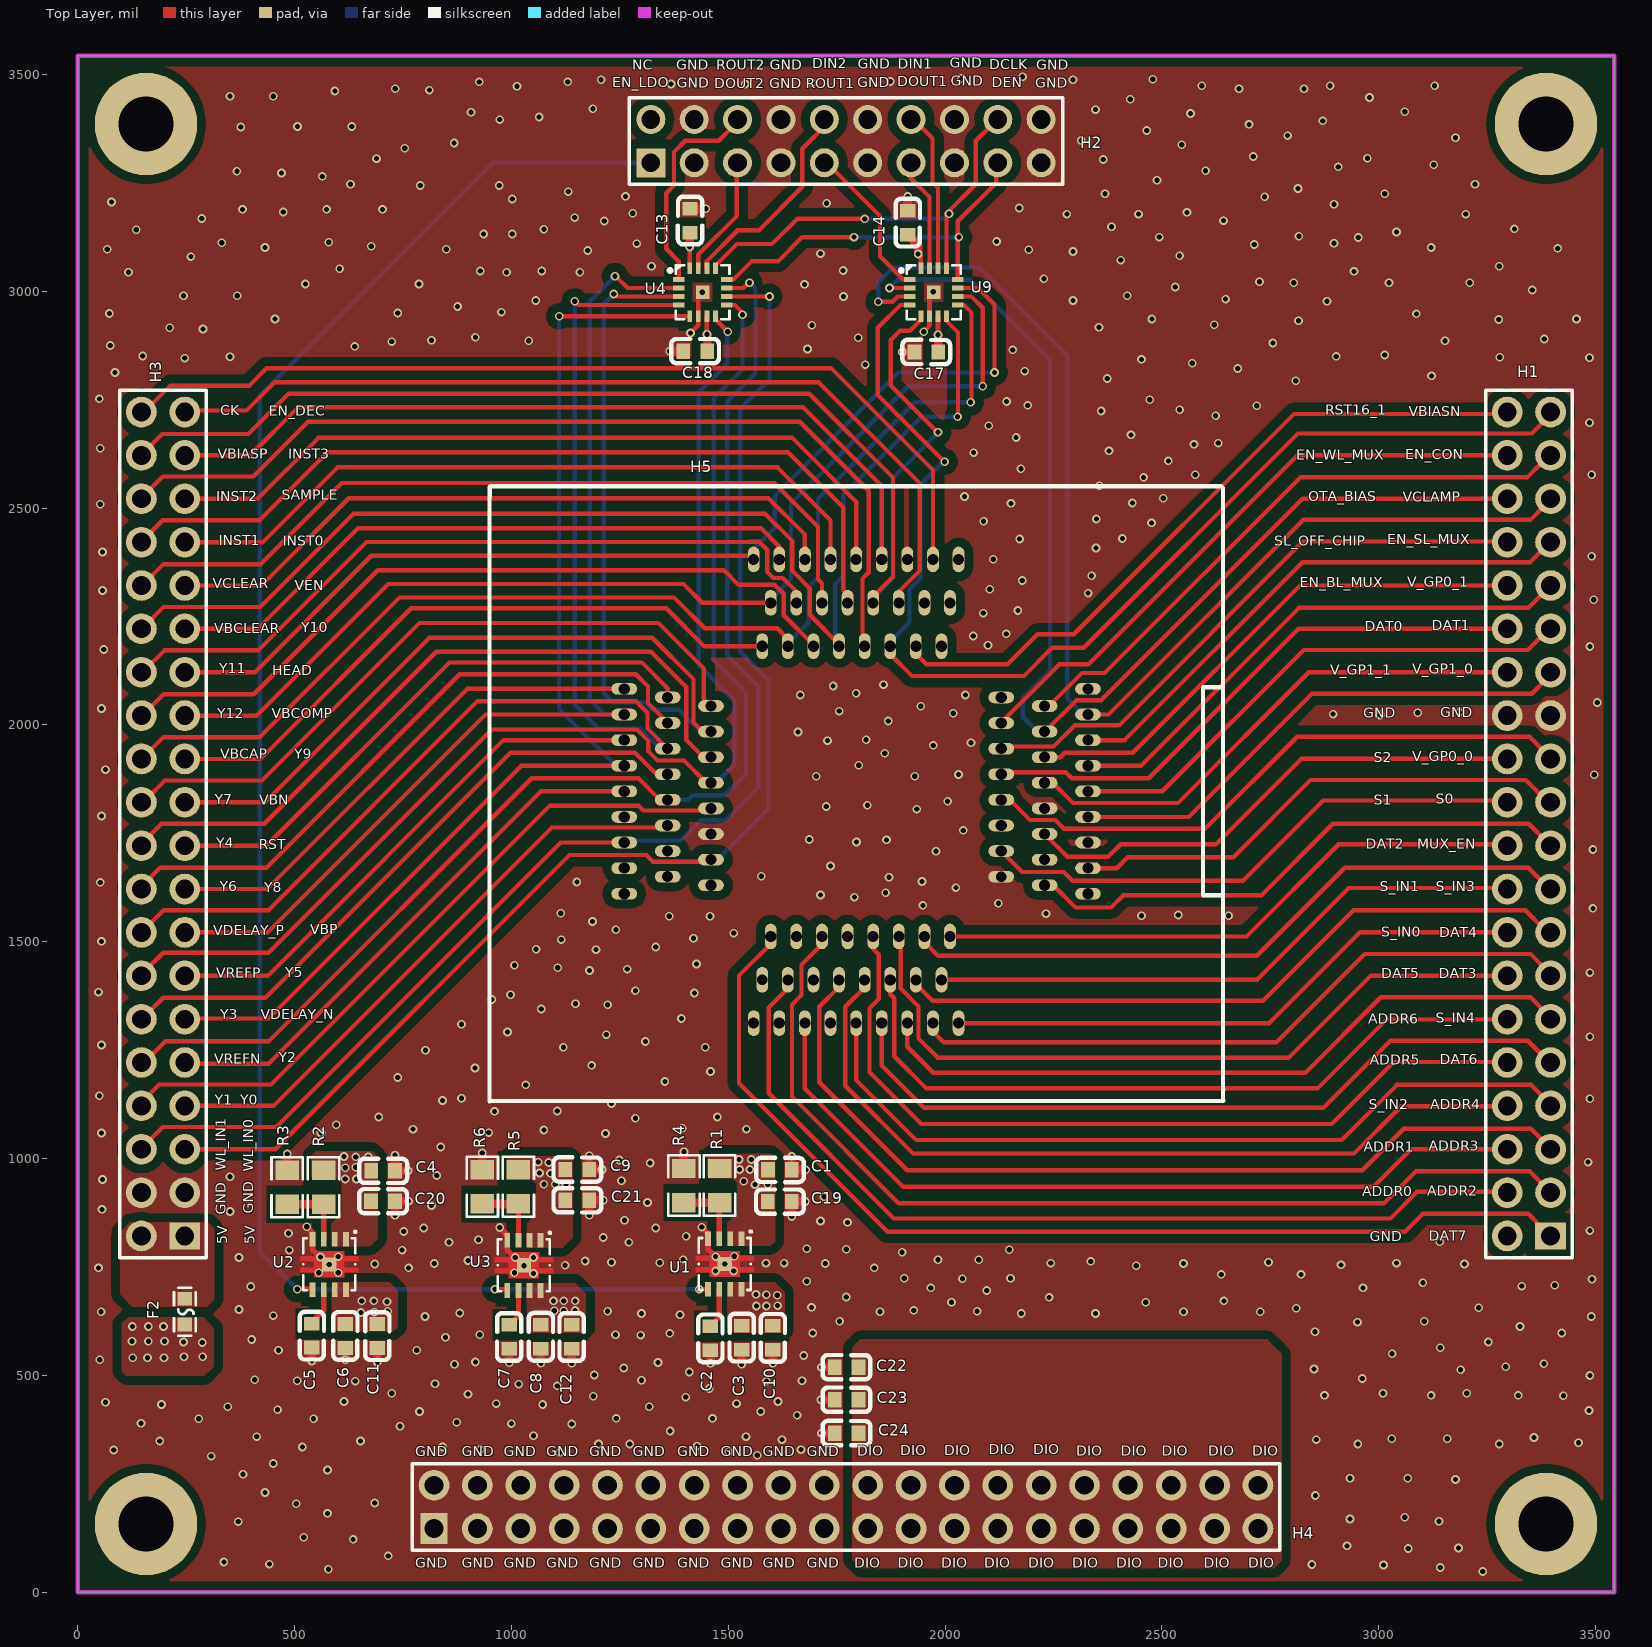
[diagram p0: Top Layer view]
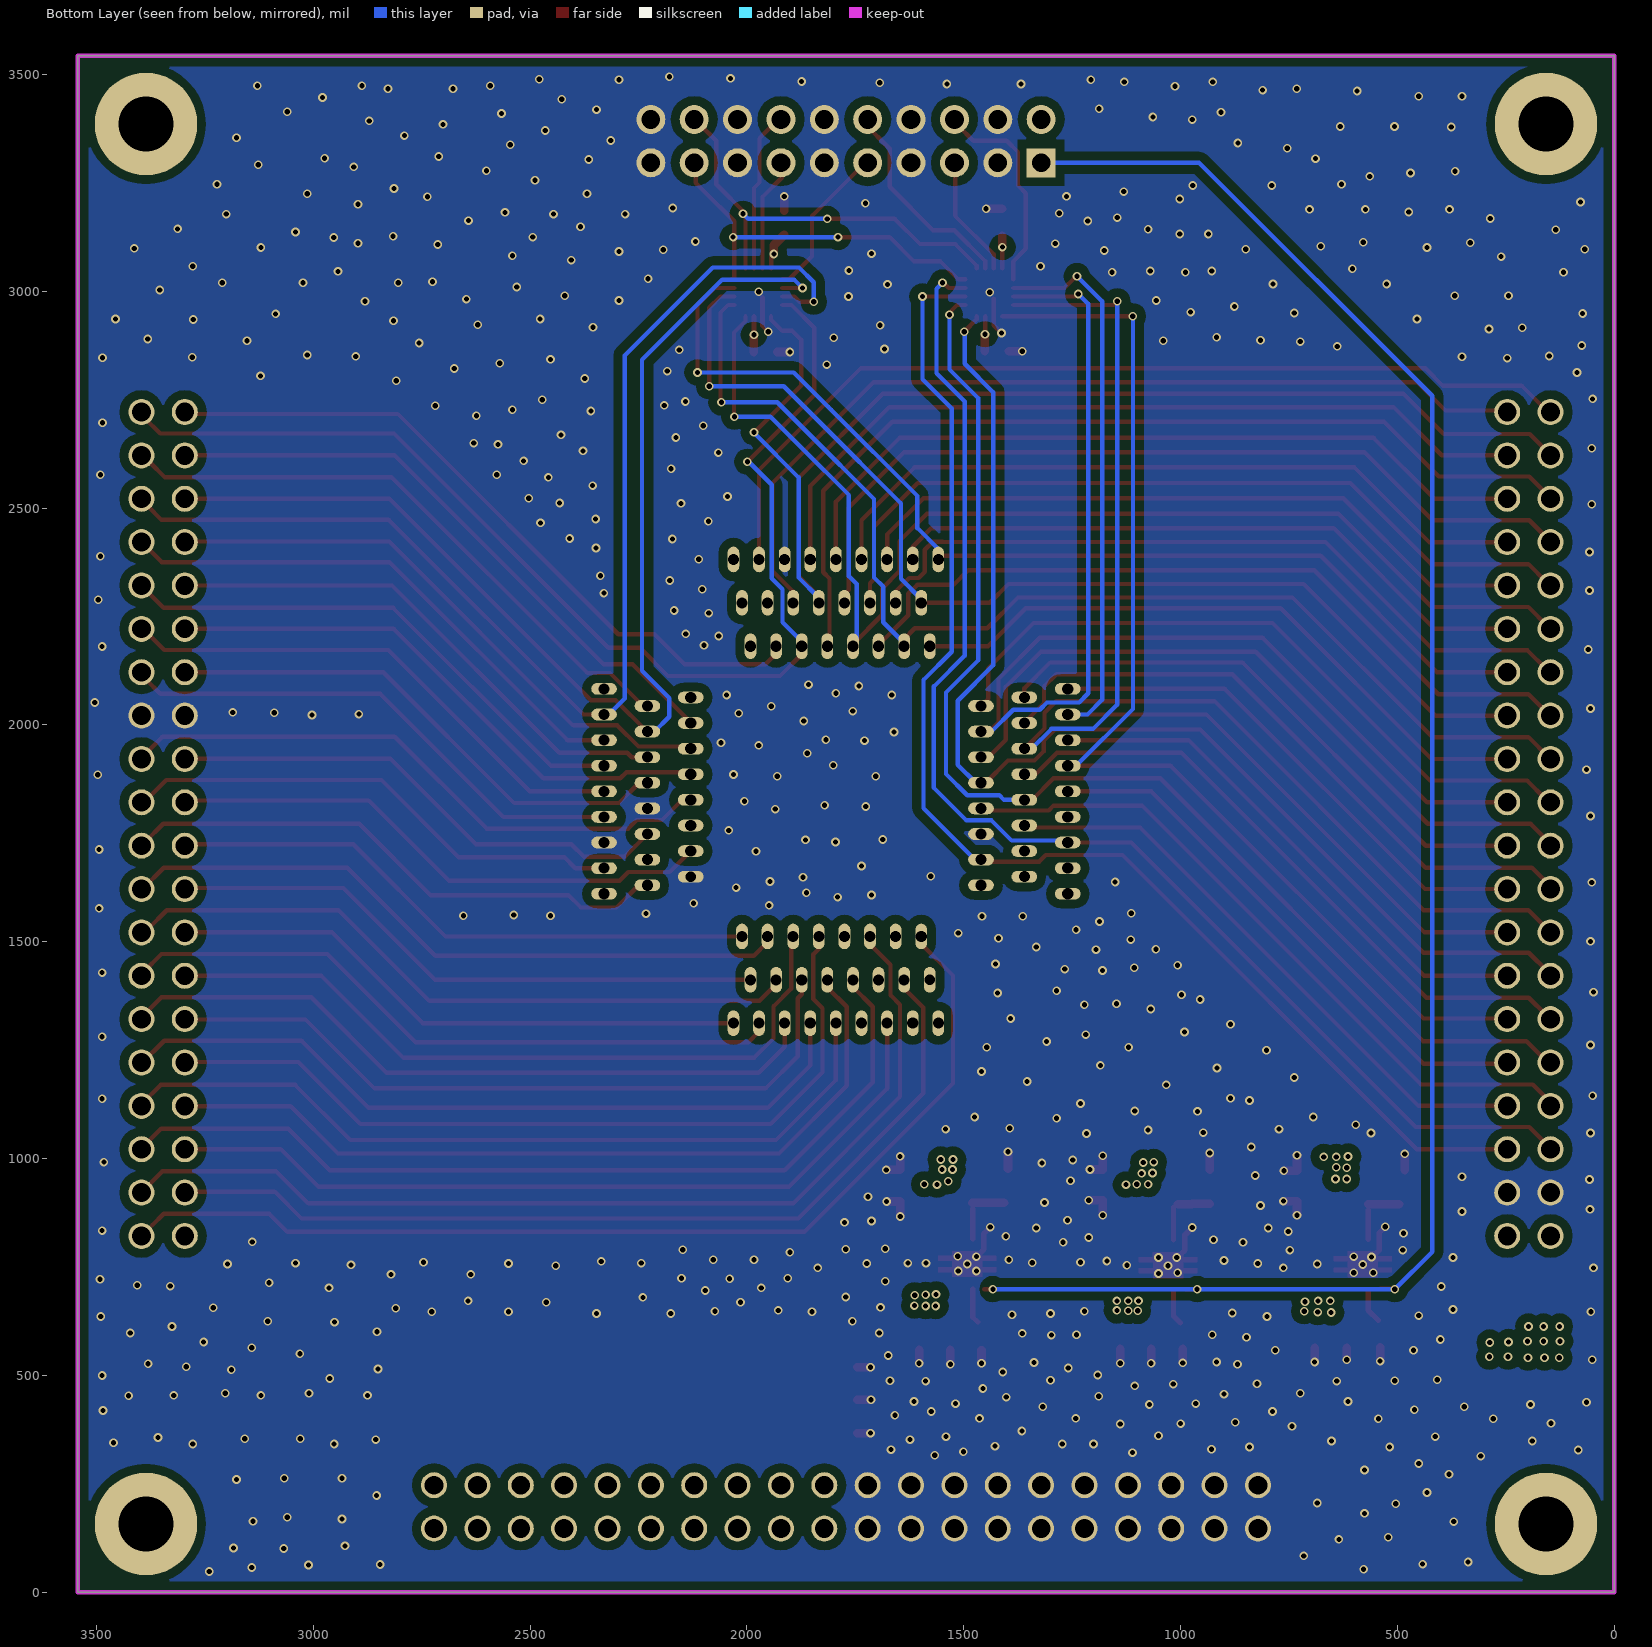
[diagram p1: Bottom Layer view, seen from below]
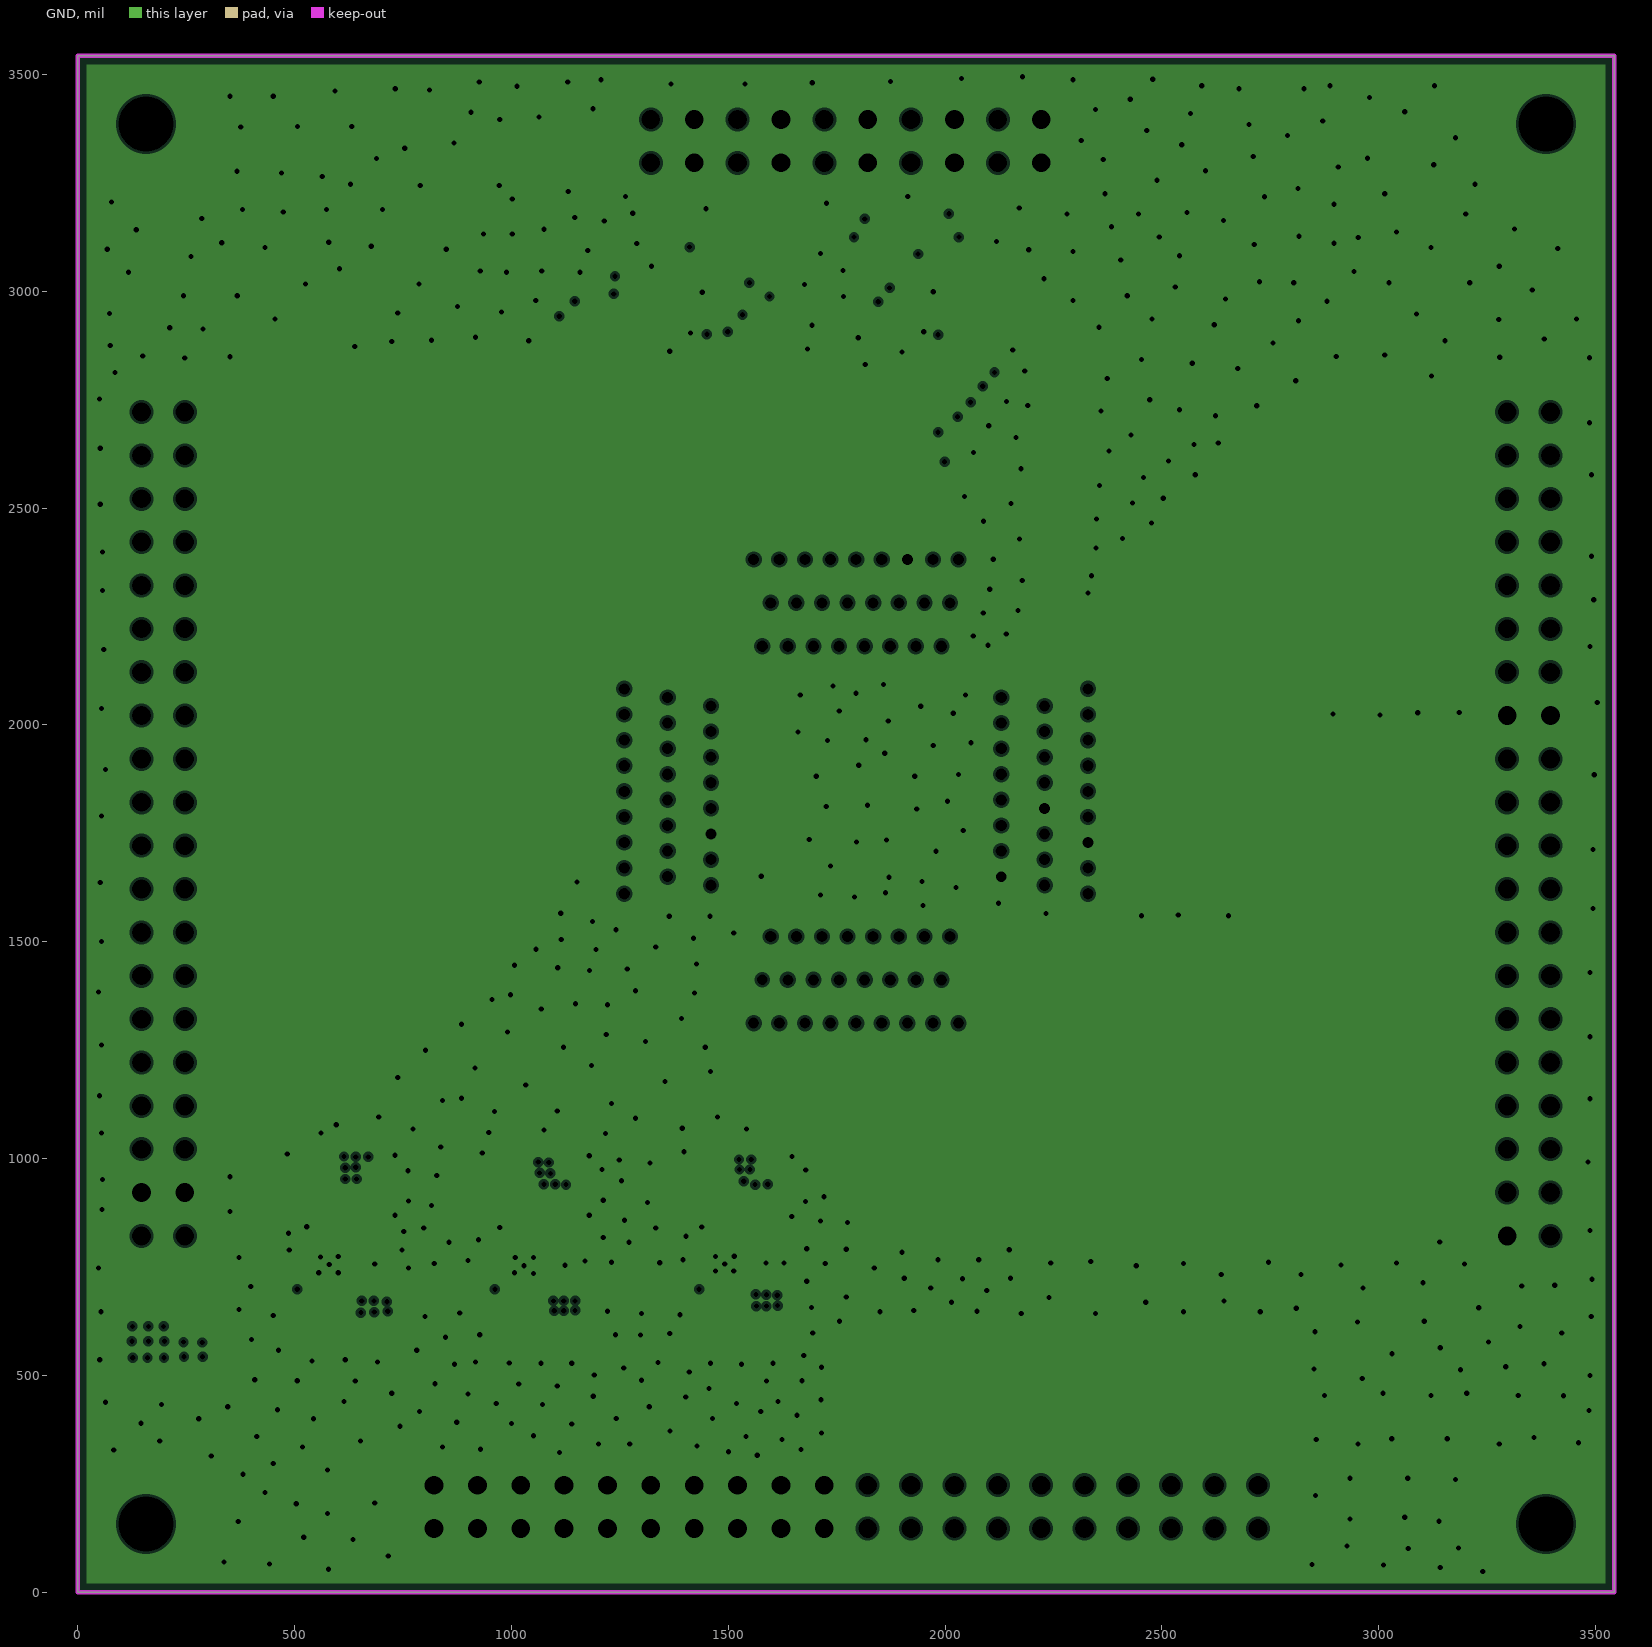
[diagram p2: GND, clearances drawn from the general rule]
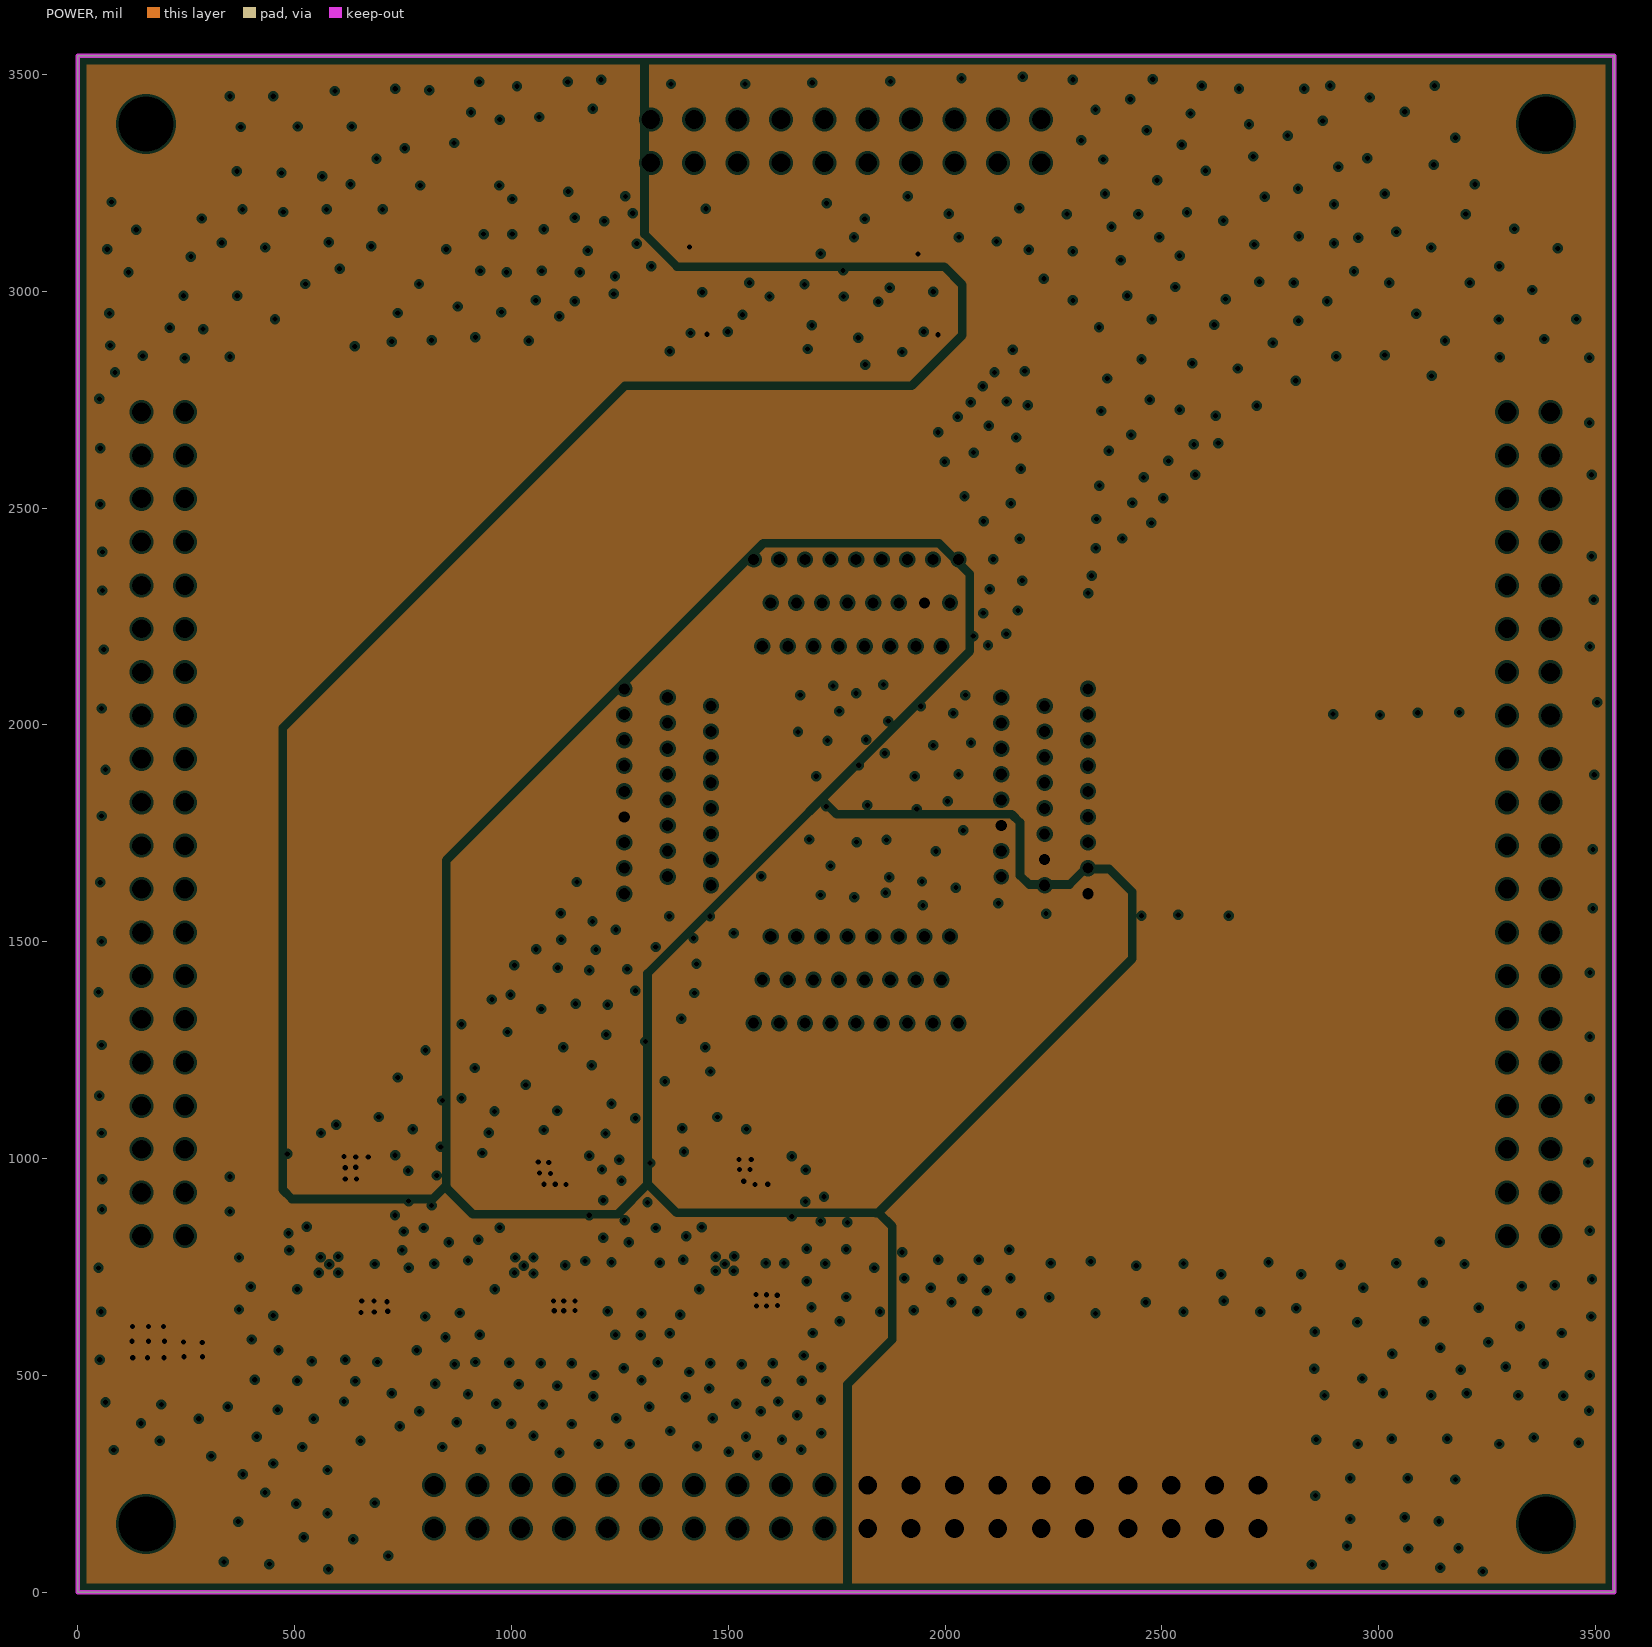
[diagram p3: POWER, clearances drawn from the general rule]
# Altium PCB MISC62795.pcbdoc (part 1 of 2)
Units mil, origin at the board's own origin, x right, y up, seen from the top; angles counter-clockwise.
Board outline 3543.31 x 3543.31 mil, 4 copper layers (Top Layer, GND, POWER, Bottom Layer); 39 components, 94 nets, 363 pads, 705 vias.

## Layer stack, top to bottom (the 12.6 mil dielectric is the usual default, probably not edited)
Top Layer: signal copper 1.4
Dielectric: core 12.6, FR-4, Dk 4.8
GND: plane copper 1.4, net GND
Dielectric: prepreg 12.6, FR-4, Dk 4.8
POWER: plane copper 1.4, net DVDDIO
Dielectric: core 12.6, FR-4, Dk 4.8
Bottom Layer: signal copper 1.4

## Board outline
0,0 3543.31,0 3543.31,3543.31 0,3543.31

## Design rules (kind name [scope] priority, off if disabled: settings)
Clearance Clearance_1 [INPOLYGON] p1: gap=6
Clearance [All] p2: gap=6
HoleSize [All] p1: absolutevalues=TRUE maxlimit=500 minlimit=1 maxpercent=80.000 minpercent=20.000
HoleToHoleClearance [All] p1: gap=0 allowstackedmicrovias=TRUE
MinimumSolderMaskSliver [All] p1: minsoldermaskwidth=0
PlaneClearance [All] p1: clearance=6
PlaneConnect [All] p1: planeconnectstyle=Direct reliefexpansion=20 reliefentries=4 reliefconductorwidth=10 reliefairgap=10
PolygonConnect [All] p1: connectstyle=Direct reliefconductorwidth=10 reliefentries=4 polygonreliefangle="90 Angle"
RoutingVias [All] p1: holewidth=12 width=20 viastyle="Through Hole" minholewidth=12 minwidth=20 maxholewidth=12 maxwidth=20
SilkToSilkClearance [All] p1: silktosilkclearance=0
SilkscreenOverComponentPads [All] p1: minsilkscreentomaskgap=0
SolderMaskExpansion [All] p1: expansion=4
Width [All] p1: maxlimit=40 minlimit=10 preferedwidth=10 minimp=50.000000 maximp=50.000000 favimp=50.000000
21 further rules are at their usual default settings.

## Components (designator, comment, footprint, x,y, rotation, side; value= is the part's Value field where it differs from the comment)
C1 "4.7uF/16V" C0603 1619.26,974.06 r180 top
C2 "10nF/16V" C0603 1459,586 r90 top
C3 "1uF/16V" C0603 1531,587 r270 top
C4 "4.7uF/16V" C0603 704.26,972.06 r180 top
C5 "10nF/16V" C0603 540,592 r90 top
C6 "1uF/16V" C0603 617,591 r270 top
C7 "10nF/16V" C0603 995,589 r90 top
C8 "1uF/16V" C0603 1068,589 r270 top
C9 "4.7uF/16V" C0603 1152,975 r180 top
C10 "4.7uF/16V" C0603 1603,587 r90 top
C11 "4.7uF/16V" C0603 691,591 r90 top
C12 "4.7uF/16V" C0603 1139,589 r90 top
C13 "0.1uF/16V" C0603 1412,3163 r270 top
C14 "0.1uF/16V" C0603 1914,3158 r270 top
C17 "0.1uF/16V" C0603 1957,2860 r0 top
C18 "0.1uF/16V" C0603 1424,2862 r0 top
C19 "4.7uF/16V" C0603 1619,901 r180 top
C20 "4.7uF/16V" C0603 704,902 r180 top
C21 "4.7uF/16V" C0603 1152,904 r180 top
C22 "4.7uF/16V" C0603 1773,519 r0 top
C23 "4.7uF/16V" C0603 1773,444 r0 top
C24 "4.7uF/16V" C0603 1773,367 r0 top
F2 "BSMD0603-050-6V" F0603 247,647 r90 top
H1 "12251220ANG0S115001" HDR-TH_40P-P2.54-V-M-R2-C20-S2.54 3346.46,1771.65 r90 top locked
H2 "PZ254V-12-20P" HDR-TH_20P-P2.54-V-M-R2-C10-S2.54 1771.65,3346.46 r0 top locked
H3 "12251220ANG0S115001" HDR-TH_40P-P2.54-V-M-R2-C20-S2.54 196.85,1771.65 r90 top locked
H4 "12251220ANG0S115001" HDR-TH_40P-P2.54-V-M-R2-C20-S2.54 1771.65,196.85 r0 top locked
H5 "220-1S-2*50PStraight row of mothersH=4.3 Gold-plated" IC51-1004-809-23 1795,1847 r90 top locked
R1 "1.25k" R0805 1480,938 r270 top
R2 "12.4k" R0805 567,934 r270 top
R3 "10k" R0805 483,934 r270 top
R4 "10k" R0805 1398,938 r270 top
R5 "12.4k" R0805 1016,935 r270 top
R6 "10k" R0805 933,935 r270 top
U1 "TPS7A8001DRBR" VSON-8_L3.0-W3.0-P0.65-TL-EP 1492,757 r270 top
U2 "TPS7A8001DRBR" VSON-8_L3.0-W3.0-P0.65-TL-EP 580,756 r270 top
U3 "TPS7A8001DRBR" VSON-8_L3.0-W3.0-P0.65-TL-EP 1029,754 r270 top
U4 "DAC60508ZRTER" WQFN-16_L3.0-W3.0-P0.50-BL-EP0.8 1441,2998 r270 top
U9 "DAC60508ZRTER" WQFN-16_L3.0-W3.0-P0.50-BL-EP0.8 1974,2998 r270 top

## Footprints (in the part's own frame and the unit in brackets; to place one, negate y for a bottom-side part, rotate by r counter-clockwise, add the part's x,y. Pads: shape width x height; smd on the part's side, far side on the other; paste and mask are expansions set on the pad)
C0603 [mm]
  rect 0.8x0.9 smd paste+0 mask+0.051: 1(-0.7,0) 2(0.7,0)
  silkscreen extent -1.41,-0.71 1.39,0.72
F0603 [mil]
  rect 31.75x34.02 smd paste-3937.01 mask+2: 1(-29.65,0) 2(29.66,0)
  silkscreen extent -55,-25 55,25
HDR-TH_20P-P2.54-V-M-R2-C10-S2.54 [mm]
  rect 1.7x1.7 hole 1.1 paste+0 mask+0.051: 1(-11.43,-1.27)
  round 1.7 hole 1.1 paste+0 mask+0.051: 2(-11.43,1.27) 3(-8.89,-1.27) 4(-8.89,1.27) 5(-6.35,-1.27) 6(-6.35,1.27) 7(-3.81,-1.27) 8(-3.81,1.27) 9(-1.27,-1.27) 10(-1.27,1.27) 11(1.27,-1.27) 12(1.27,1.27) 13(3.81,-1.27) 14(3.81,1.27) 15(6.35,-1.27) 16(6.35,1.27) 17(8.89,-1.27) 18(8.89,1.27) 19(11.43,-1.27) 20(11.43,1.27)
  silkscreen extent -12.7,-2.54 12.7,2.54
HDR-TH_40P-P2.54-V-M-R2-C20-S2.54 [mm]
  rect 1.575x1.8 / inner round 1.524 / far side round 1.524 hole 1.1: 1(-24.13,-1.27)
  round 1.8 / inner round 1.524 / far side round 1.524 hole 1.1: 2(-24.13,1.27) 3(-21.59,-1.27) 4(-21.59,1.27) 5(-19.05,-1.27) 6(-19.05,1.27) 7(-16.51,-1.27) 8(-16.51,1.27) 9(-13.97,-1.27) 10(-13.97,1.27) 11(-11.43,-1.27) 12(-11.43,1.27) 13(-8.89,-1.27) 14(-8.89,1.27) 15(-6.35,-1.27) 16(-6.35,1.27) 17(-3.81,-1.27) 18(-3.81,1.27) 19(-1.27,-1.27) 20(-1.27,1.27) 21(1.27,-1.27) 22(1.27,1.27) 23(3.81,-1.27) 24(3.81,1.27) 25(6.35,-1.27) 26(6.35,1.27) 27(8.89,-1.27) 28(8.89,1.27) 29(11.43,-1.27) 30(11.43,1.27) 31(13.97,-1.27) 32(13.97,1.27) 33(16.51,-1.27) 34(16.51,1.27) 35(19.05,-1.27) 36(19.05,1.27) 37(21.59,-1.27) 38(21.59,1.27) 39(24.13,-1.27) 40(24.13,1.27)
  silkscreen extent -25.4,-2.54 25.4,2.54
IC51-1004-809-23 [mm] "测试座"
  oval 1.5x0.686 hole 0.65: 1(-13.58,6) 3(-8.5,5) 4(-13.58,4.5) 5(-11.04,4) 6(-8.5,3.5) 7(-13.58,3) 8(-11.04,2.5) 9(-8.5,2) 10(-13.58,1.5) 11(-11.04,1) 12(-8.5,0.5) 13(-13.58,0) 14(-11.04,-0.5) 15(-8.5,-1) 16(-13.58,-1.5) 17(-11.04,-2) 18(-8.5,-2.5) 19(-13.58,-3) 20(-11.04,-3.5) 21(-8.5,-4) 22(-13.58,-4.5) 23(-11.04,-5) 24(-8.5,-5.5) 25(-13.58,-6) 51(13.58,-6) 52(11.04,-5.5) 53(8.5,-5) 54(13.58,-4.5) 55(11.04,-4) 56(8.5,-3.5) 57(13.58,-3) 58(11.04,-2.5) 59(8.5,-2) 60(13.58,-1.5) 61(11.04,-1) 62(8.5,-0.5) 63(13.58,0) 64(11.04,0.5) 65(8.5,1) 66(13.58,1.5) 67(11.04,2) 68(8.5,2.5) 69(13.58,3) 70(11.04,3.5) 71(8.5,4) 72(13.58,4.5) 73(11.04,5) 74(8.5,5.5) 75(13.58,6)
  oval 1.5x0.686 hole 0.61: 2(-11.04,5.5)
  oval 0.686x1.5 hole 0.65: 26(-6,-13.58) 27(-5.5,-11.04) 29(-4.5,-13.58) 30(-4,-11.04) 31(-3.5,-8.5) 32(-3,-13.58) 33(-2.5,-11.04) 34(-2,-8.5) 35(-1.5,-13.58) 36(-1,-11.04) 37(-0.5,-8.5) 38(0,-13.58) 39(0.5,-11.04) 40(1,-8.5) 41(1.5,-13.58) 42(2,-11.04) 43(2.5,-8.5) 44(3,-13.58) 45(3.5,-11.04) 46(4,-8.5) 47(4.5,-13.58) 48(5,-11.04) 49(5.5,-8.5) 50(6,-13.58) 76(6,13.58) 77(5.5,11.04) 78(5,8.5) 79(4.5,13.58) 80(4,11.04) 81(3.5,8.5) 82(3,13.58) 83(2.5,11.04) 84(2,8.5) 85(1.5,13.58) 86(1,11.04) 87(0.5,8.5) 88(0,13.58) 89(-0.5,11.04) 90(-1,8.5) 91(-1.5,13.58) 92(-2,11.04) 93(-2.5,8.5) 94(-3,13.58) 95(-3.5,11.04) 96(-4,8.5) 97(-4.5,13.58) 98(-5,11.04) 99(-5.5,8.5) 100(-6,13.58)
  oval 0.686x1.5 hole 0.61: 28(-5,-8.5)
  silkscreen extent -18.16,-21.49 17.87,21.48
R0805 [mil]
  rect 44.59x54.21 smd paste-3937.01 mask+2: 1(-39.37,0) 2(39.37,0)
  silkscreen extent -69,-36 69,36
VSON-8_L3.0-W3.0-P0.65-TL-EP [mm]
  rect 0.85x0.34 smd paste+0 mask+0.051: 1(-1.476,0.975) 2(-1.476,0.325) 3(-1.476,-0.325) 4(-1.476,-0.975) 5(1.476,-0.975) 6(1.476,-0.325) 7(1.476,0.325) 8(1.476,0.975)
  rect 0.838x0.838 smd paste+0 mask+0.051: 9(0,0)
  Top Layer region: -0.76,0.89 -0.47,0.89 -0.47,1.71 -0.18,1.71 -0.18,0.88 0.18,0.88 0.18,1.71 0.47,1.71 0.47,0.88 0.76,0.88 0.76,-0.89 0.47,-0.89 0.47,-1.71 0.18,-1.71 0.18,-0.89 -0.18,-0.89 -0.18,-1.71 -0.47,-1.71 -0.47,-0.89 -0.76,-0.89 -0.76,0.89
  silkscreen extent -1.96,-1.52 1.52,1.58
WQFN-16_L3.0-W3.0-P0.50-BL-EP0.8 [mm]
  rect 0.28x0.665 smd paste+0 mask+0.051: 1(-0.75,-1.407) 2(-0.25,-1.407) 3(0.25,-1.407) 4(0.75,-1.407) 9(0.75,1.407) 10(0.25,1.407) 11(-0.25,1.407) 12(-0.75,1.407)
  rect 0.665x0.28 smd paste+0 mask+0.051: 5(1.407,-0.75) 6(1.407,-0.25) 7(1.407,0.25) 8(1.407,0.75) 13(-1.407,0.75) 14(-1.407,0.25) 15(-1.407,-0.25) 16(-1.407,-0.75)
  rect 0.8x0.8 smd paste+0 mask+0.051: 17(0,0)
  silkscreen extent -1.58,-2 1.58,1.58

## Part data
C1 C4 C9 C10 C11 C12 C19 C20 C21 C22 C23 C24: library part 4.7uF
C2 C5 C7 C13 C14 C17 C18: library part 10nF
C3 C6 C8: library part 1uF

## Free pads (board coordinates)
  round 236.22 hole 125.98: 0(157.48,157.48) 0(157.48,3385.83) 0(3385.83,157.48) 0(3385.83,3385.83)

## Via types
v1: diameter 20, hole 12, Top Layer to Bottom Layer, 705 vias

## Nets (pads, with @x,y where several pads share a name; then routed paths per layer and width w, separated by ;. In a path a pad name is that pad's centre, name@x,y a point inside that pad or via, vN(x,y) a via of type N, cw(c..) or ccw(c..) an arc to the next point about the centre after c; other vN are vias at no path point)
5.0V: F2.2 H3.1 H3.2
5V: C3.1 C6.1 C8.1 C10.2 C11.2 C12.2 C17.2 C18.2 F2.1 U1.7 U1.8 U2.7 U2.8 U3.7 U3.8 U4.7 U9.7 | length 163.7
  Top Layer w10.5: v1@1450.84,2899 v1@1450.84,2901 ; U4.7@1450.84,2942.59 v1@1450.84,2901 ; v1(1451,2901) v1@1450.84,2901 ; v1@1983.84,2898.45 v1@1983.84,2900 ; U9.7@1983.84,2942.59 v1@1983.84,2900 ; v1(1984,2900) v1@1983.84,2900
  Top Layer w20: v1@1451,2899 1451.55,2898.45 C18.2@1451.55,2862 ; C17.2@1984.55,2860 v1@1984.55,2898.45
  other v1: 127,541 161,541 199,541 245,543 288,543 287,576 244,577 125,579 163,579 200,579 126,613 163,613 198,613 653,645 684,646 715,648 1099,649 1121,649 1147,650 1565,660 1588,660 1614,661 713,670 655,672 683,672 1097,672 1121,672 1147,672 1613,685 1588,686 1564,687
ARRAY_ADDR0: H1.4 H5.5 | length 2143.6
  Top Layer w10: H5.5@1637.52,1412.35 1637.52,1392.52 1593.33,1348.33 1593.33,1150.67 1882,862 3027,862 3089,924 3217,924 ; 3242,924 3217,924 ; H1.4@3285,920 3281,924 3217,924
ARRAY_ADDR1: H1.6 H5.7 | length 1940.9
  Top Layer w10: H5.7@1676.89,1312.35 1676.89,1161.11 1903,935 2988,935 3075,1022 3202,1022 ; 3244,1022 3202,1022 ; H1.6@3294,1020 3292,1022 3202,1022
ARRAY_ADDR2: H1.3 H5.9 | length 2295.2
  Top Layer w10: H5.9@1716.26,1512.35 1716.26,1494.26 1669,1447 1669,1377 1647,1355 1647,1143 1893,897 3012,897 3086,971 3343,971 3348,971 H1.3@3393,926
ARRAY_ADDR3: H1.5 H5.11 | length 2082.3
  Top Layer w10: H5.11@1755.63,1412.35 1755.63,1395.63 1710,1350 1710,1176 1913,973 2962,973 3058,1069 3351,1069 H1.5@3395,1025
ARRAY_ADDR4: H1.7 H5.13 | length 1858.9
  Top Layer w10: H5.13@1795,1312.35 1795,1181 1933,1043 2915,1043 3042,1170 3352,1170 H1.7@3395,1127
ARRAY_ADDR5: H1.10 H5.15 | length 1928.1
  Top Layer w10: H5.15@1834.37,1512.35 1834.37,1483.63 1847,1471 1847,1368 1826,1347 1826,1199 1945,1080 2892,1080 3035,1223 3214,1223 ; 3240,1223 3214,1223 ; H1.10@3291,1220 3288,1223 3214,1223
ARRAY_ADDR6: H1.12 H5.17 | length 1844.7
  Top Layer w10: H5.17@1873.74,1412.35 1873.74,1379.26 1883,1370 1883,1236 1957,1162 2859,1162 3018,1321 3084,1321 ; 3250.02,1321 3084,1321 ; H1.12@3285,1321 3084,1321
ARRAY_DAT0: H1.30 H5.40 | length 1318
  Top Layer w10: H5.40@2129.65,1886.37 2134.46,1891.19 2277.81,1891.19 2292,1877 2470,1877 2814.65,2221.65 H1.30@3296.46,2221.65 ; H1.30@3296.46,2224 H1.30@3297,2224
ARRAY_DAT1: H1.29 H5.38 | length 1194.6
  Top Layer w10: H5.38@2329.65,1847 2501,1847 2827,2173 3344,2173 H1.29@3376,2205
ARRAY_DAT2: H1.20 H5.24 | length 1381.5
  Top Layer w10: H5.24@2011.54,1512.35 2695.35,1512.35 2908,1725 3228,1725 ; 3244,1725 3228,1725 ; H1.20@3289,1725 3228,1725
ARRAY_DAT3: H1.13 H5.22 | length 1550.1
  Top Layer w10: H5.22@1972.17,1312.35 1972.17,1292.83 1997,1268 2764,1268 2968,1472 3350,1472 H1.13@3391,1431
ARRAY_DAT4: H1.15 H5.20 | length 1577.1
  Top Layer w10: H5.20@1932.8,1412.35 1932.8,1402.2 1971,1364 2733,1364 2942,1573 3338,1573 H1.15@3380,1531
ARRAY_DAT5: H1.14 H5.18 | length 1701.7
  Top Layer w10: H5.18@1893.43,1512.35 1898.24,1507.54 1898.24,1391.76 1939,1351 1939,1277 1983,1233 2793,1233 2982,1422 H1.14@3290,1422
ARRAY_DAT6: H1.9 H5.16 | length 1765.7
  Top Layer w10: H5.16@1854.05,1312.35 1854.05,1214.95 1952,1117 2872,1117 3027,1272 3344,1272 H1.9@3396,1220
ARRAY_DAT7: H1.1 H5.3 | length 2386.3
  Top Layer w10: H5.3@1598.15,1512.35 1598.15,1495.15 1525,1422 1525,1174 1868,831 3060,831 3102,873 3345,873 H1.1@3372,846
ARRAY_INST0: H3.33 H5.66 | length 1904.7
  Top Layer w10: H3.33@246.85,2421.65 H3.33@269,2421.65 ; H3.33@269,2421 426,2421 599,2594 933,2594 ; 730,2594 933,2594 ; H5.66@1735.94,2381.65 1735.94,2472.06 1614,2594 933,2594
ARRAY_INST1: H3.34 H5.64 | length 2002.5
  Top Layer w10: H3.34@157,2433 196,2472 419,2472 576,2629 785,2629 ; 727,2629 785,2629 ; H5.64@1774,2303 1765,2312 1765,2502 1638,2629 785,2629
ARRAY_INST2: H3.36 H5.62 | length 2170.2
  Top Layer w10: H3.36@155,2532 196,2573 405,2573 531,2699 1665,2699 1824,2540 1824,2352 1809.87,2337.87 1809.87,2186.46 H5.62@1814.68,2181.65
ARRAY_INST3: H3.37 H5.60 | length 1897.9
  Top Layer w10: H3.37@246.85,2621.65 H3.37@252,2621.65 ; H3.37@252,2622 398,2622 509,2733 1672,2733 1854.05,2550.95 H5.60@1854.05,2381.65
AVDD: C9.2 C21.2 H5.55 H5.91 R5.1 U3.1 U3.2
  other v1: 1126,940 1075,941 1101,941 1090,966 1065,967 1086,991 1062,992
CK: H3.40 H5.54 | length 2153.3
  Top Layer w10: H3.40@161,2730 213,2782 395,2782 436,2823 1737,2823 1972.17,2587.83 H5.54@1972.17,2381.65
DAC_CLK: H2.18 U4.13 U9.13 | length 967.9
  Top Layer w10: U4.13@1470.53,3053.41 1470.53,3059.53 1520,3109 1601,3109 1659,3167 v1(1815,3167) ; U9.13@2003.53,3053.41 2003.53,3179.53 2071,3247 2071,3347 H2.18@2108,3384
  Bottom Layer w10: v1(1815,3167) 1997,3167 v1(2009,3179)
DAC_DATA_OUT1: H2.13 U9.15 | length 262.7
  Top Layer w10: H2.13@1920,3288 1920,3262 1964.16,3217.84 1964.16,3136 ; U9.15@1964.16,3053.41 1964.16,3136 ; 1964.16,3145.84 1964.16,3136
DAC_DATA_OUT2: H2.5 U4.15 | length 267.4
  Top Layer w10: U4.15@1431.16,3053.41 1431.16,3085.16 1520,3174 H2.5@1520,3284
DAC_EN: H2.17 U4.12 U9.12 | length 886
  Top Layer w10: U4.12@1496.41,3027.53 1512.53,3027.53 1554,3069 1615,3069 1671,3125 v1(1790,3125) ; U9.12@2036,3027.53 U9.12@2029.41,3027.53 2029.41,3161.41 2096,3228 ; 2104,3236 2096,3228 ; H2.17@2118,3283 2118,3250 2096,3228
  Bottom Layer w10: v1(1790,3125) v1(2032,3125)
DAC_IN1: H2.14 U9.14 | length 371.5
  Top Layer w10: H2.14@1929,3395 1971,3353 1971,3251 1983.84,3238.16 1983.84,3167 ; U9.14@1983.84,3053.41 1983.84,3167 ; 1983.84,3174.16 1983.84,3167
DAC_IN2: H2.10 U4.14 | length 477.5
  Top Layer w10: U4.14@1450.84,3053.41 1450.84,3069.84 1522,3141 1571,3141 1671,3241 1671,3329 H2.10@1729,3387
DAC_REF_OUT1: H2.9 U9.1 | length 333.6
  Top Layer w10: H2.9@1744,3280 1850,3174 1850,3081 1903.47,3027.53 U9.1@1918.59,3027.53
DAC_REF_OUT2: H2.6 U4.1 | length 474.6
  Top Layer w10: U4.1@1385.59,3027.53 1385.59,3069.41 1357,3098 1357,3226 1375,3244 1375,3321 1401,3347 1478,3347 H2.6@1512,3381
DVDD: C1.2 C19.2 H5.26 H5.34 R1.1 U1.1 U1.2
  other v1: 1562,940 1591,941 1536,948 1526,975 1550,975 1525,998 1553,998
DVDDIO: C4.2 C13.2 C14.2 C20.2 C22.2 C23.2 C24.2 H4.21 H4.22 H4.23 H4.24 H4.25 H4.26 H4.27 H4.28 H4.29 H4.30 H4.31 H4.32 H4.33 H4.34 H4.35 H4.36 H4.37 H4.38 H4.39 H4.40 H5.30 R2.1 U2.1 U2.2 U4.16 U9.16 | length 161.2
  Top Layer w10.5: v1(1411,3102) 1411.47,3102 U4.16@1411.47,3053.41 ; v1(1938,3086) 1944.47,3079.53 U9.16@1944.47,3053.41
  Top Layer w20: v1@1411.47,3102 C13.2@1411.47,3128.53 ; C14.2@1914,3130.45 1938,3106.45 v1@1938,3090
  other v1: 617,953 643,953 617,979 641,980 641,1004 670,1004 614,1005
EN_BL_MUX: H1.32 H5.42 | length 1230.8
  Top Layer w10: H5.42@2229.65,1925.74 2265.74,1925.74 2276,1936 2433,1936 2818.65,2321.65 H1.32@3296.46,2321.65
EN_CON: H1.37 H5.48 | length 1380.2
  Top Layer w10: H5.48@2229.65,2043.85 2239.6,2043.85 2315.75,2120 2368,2120 2819,2571 3342,2571 H1.37@3377,2606
EN_DEC: H3.39 H5.58 | length 2113.5
  Top Layer w10: H3.39@246.85,2721.65 H3.39@260,2721.65 ; H3.39@260,2725 389,2725 454,2790 1709,2790 1942,2557 1942,2356 1894,2308 H5.58@1894,2299 ; H5.58@1893.43,2281.65 1893.43,2296.43 H5.58@1895,2298
EN_LDO: H2.1 U1.5 U2.5 U3.5 | length 4226.9
  Top Layer w10: v1@507,700 U2.5@540,700 ; v1(962,699) U3.5@989,699 ; v1(1433,699) U1.5@1453,699
  Bottom Layer w10: H2.1@1321.65,3296.46 957.46,3296.46 420,2759 420,2397 420,2395 420,785 v1(506,699) v1(962,699) v1(1433,699)
EN_SL_MUX: H1.33 H5.44 | length 1240
  Top Layer w10: H5.44@2329.65,1965.11 2414.11,1965.11 2824,2375 2843,2375 ; 2843,2375.22 3349.22,2375.22 H1.33@3385,2411
EN_WL_MUX: H1.38 H5.46 | length 1442.2
  Top Layer w10: H5.46@2129.65,2004.48 H5.46@2138.48,2004.48 ; H5.46@2132,2008 2264,2140 2331,2140 2813,2622 3219,2622 ; 3240,2622 3219,2622 ; H1.38@3290,2622 3219,2622
GND: C1.1 C2.1 C3.2 C4.1 C5.1 C6.2 C7.1 C8.2 C9.1 C10.1 C11.1 C12.1 C13.1 C14.1 C17.1 C18.1 C19.1 C20.1 C21.1 C22.1 C23.1 C24.1 H1.2 H1.25 H1.26 H2.3 H2.4 H2.7 H2.8 H2.11 H2.12 H2.15 H2.16 H2.19 H2.20 H3.3 H3.4 H4.1 H4.2 H4.3 H4.4 H4.5 H4.6 H4.7 H4.8 H4.9 H4.10 H4.11 H4.12 H4.13 H4.14 H4.15 H4.16 H4.17 H4.18 H4.19 H4.20 H5.28 H5.32 H5.36 H5.57 H5.93 R3.1 R4.1 R6.1 U1.4 U1.9 U2.4 U2.9 U3.4 U3.9 U4.6 U4.17 U9.6 U9.17 | length 1408.9
  Top Layer w10: H5.36@2229.65,1807.63 H5.36@2253.37,1807.63
  Top Layer w10.5: v1(1413,2904) 1431.16,2922.16 U4.6@1431.16,2942.59 U4.17@1431.16,2983.16 ; v1(1951,2907) 1964.16,2920.16 U9.6@1964.16,2942.59 U9.17@1964.16,2985.84
  Top Layer w13: v1(528,843) 541.6,829.4 U2.4@541.6,814.1 541.6,789.4 548,783 ; v1(973,841) 990.6,823.4 U3.4@990.6,812.1 990.6,788.4 997,782 ; v1(1439,842) 1453.6,827.4 U1.4@1453.6,815.1 1453.6,790.4 1460,784
  Top Layer w20: R3.1@483,973.37 v1(483,1011) ; v1(540,533) C5.1@540,564.45 ; v1(617,536) C6.2@617,563.45 ; v1(691,531) C11.1@691,563.45 ; v1(731.55,869.45) C20.1@731.55,902 v1(763,902) ; v1(731.81,1007.81) C4.1@731.81,972.06 v1(761.94,972.06) ; R6.1@933,974.37 v1(933,1013) ; v1(995,529) C7.1@995,561.45 ; v1(1068,528) C8.2@1068,561.45 ; v1(1139,528) C12.1@1139,561.45 ; v1(1179.55,869.56) C21.1@1179.55,904 v1(1212,904) ; v1(1179.55,1006.56) C9.1@1179.55,975 v1(1209,975) ; v1(1365,2862) C18.1@1396.45,2862 ; R4.1@1398,977.37 v1(1398,1016) ; C13.1@1412,3190.55 v1(1448.55,3190.55) ; v1(1459,528) C2.1@1459,558.45 ; v1(1531,526) C3.2@1531,559.45 ; v1(1603,528) C10.1@1603,559.45 ; v1(1646.55,866.45) C19.1@1646.55,901 v1(1678,901) ; v1(1646.81,1005.19) C1.1@1646.81,974.06 v1(1679.06,974.06) ; v1(1714,444) C23.1@1745.45,444 ; v1(1715,367) C24.1@1745.45,367 ; v1(1715,519) C22.1@1745.45,519 ; v1(1901,2860) C17.1@1929.45,2860 ; C14.1@1914,3185.55 v1(1914,3219)
  other v1: 3240,48 578,53 3142,57 3011,63 2846,64 442,65 337,70 716,84 3068,101 3184,102 2927,107 635,122 521,127 370,163 3139,164 2934,169 3060,173 576,182 504,204 685,206 2854,223 432,230 3177,260 2934,263 3067,263 381,272 576,282 451,297 308,314 1567,316 1111,322 1501,324 83,328 1668,329 929,330 518,335 841,335 1428,337 1201,342 1273,342 2952,342 3278,342 3461,345 189,349 652,349 1624,352 2856,352 3030,354 3158,354 3358,357 413,359 1541,359 1051,361 1366,372 743,383 1139,388 1000,389 146,390 874,392 279,400 544,400 1242,401 1464,401 1659,408 788,417 1575,417 3485,419 461,421 346,428 1318,428 193,433 1072,433 965,435 1519,435 64,438 614,440 1615,440 1402,450 1189,452 3426,453 2875,454 3121,454 3322,454 900,457 724,459 3010,459 3203,459 1456,470 1106,476 1017,480 824,481 640,487 1588,487 506,488 1670,488 1300,489 408,490 2962,493 3487,500 1191,501 1410,508 3189,513 2851,515 1259,517 3293,520 869,526 3381,527 1338,530 917,531 51,536 1674,546 3031,550 463,558 782,558 3142,564 3253,577 401,583 848,588 1298,593 927,594 1240,594 1365,597 1695,598 3422,598 2853,601 3326,613 2951,623 1757,625 3105,625 801,636 3490,636 451,638 1389,640 1300,643 2176,643 2347,643 881,644 54,647 1850,647 2550,647 2727,647 1222,648 2074,648 1928,650 372,652 2810,655 3231,656 1692,657 2015,669 2463,669 2643,672 2240,680 1772,681 2096,696 1967,702 2964,702 399,705 3330,706 3406,708 3102,714 1681,717 3492,722 2040,723 1906,724 2151,724 2637,733 2821,733 1051,735 556,737 601,737 1007,737 1471,741 1513,741 48,748 763,748 1837,748 1029,753 2441,753 1124,754 2913,755 580,756 685,757 1492,757 3198,757 822,758 1724,758 2550,758 1587,759 1629,759 2244,759 3041,759 1342,760 1231,761 2746,761 2336,763 1170,764 900,765 1396,767 1984,767 2078,767 372,772 1009,772 1051,772 560,773 601,774 1471,774 1514,775 1901,784 488,789 748,789 2148,790 1772,791 1681,792 856,807 1271,807 3141,808 924,813 1212,818 1403,821 486,828 752,832 3487,834 798,840 1333,840 1775,853 1713,856 1261,858 351,878 56,883 816,892 1314,899 1721,912 1254,949 57,952 351,958 828,961 1320,990 3483,992 1249,997 837,1027 1217,1058 55,1059 561,1059 948,1060 1075,1066 773,1068 1542,1068 1394,1070 596,1078 1286,1093 694,1096 1475,1096 961,1109 1106,1110 1231,1127 841,1134 3487,1138 885,1139 50,1145 1033,1170 1354,1178 738,1187 1459,1201 916,1209 1185,1215 802,1250 1120,1257 1447,1257 55,1262 1309,1270 3487,1281 1219,1286 991,1292 885,1310 1392,1323 1069,1345 1222,1355 1148,1357 955,1367 998,1378 1422,1382 48,1384 1286,1387 3487,1429 1180,1434 1267,1437 1107,1440 1007,1446 1427,1449 1195,1482 1057,1483 1333,1488 55,1501 1115,1505 1420,1508 1513,1520 1241,1528 1187,1547 1364,1559 1458,1559 2453,1560 2654,1560 2538,1562 2233,1565 1114,1566 3494,1577 1949,1584 2123,1589 1791,1603 1713,1608 1863,1613 2025,1625 52,1637 1151,1638 1947,1639 1871,1649 1576,1651 1736,1675 1979,1709 3494,1713 1796,1730 1865,1735 1687,1736 2042,1757 55,1790 1935,1806 1726,1812 1821,1815 2006,1824 1703,1882 1930,1882 3497,1885 2031,1886 64,1897 1801,1907 1861,1935 1973,1953 2060,1959 1729,1964 1818,1966 1661,1984 1869,2009 3003,2023 2895,2025 2019,2027 3090,2028 3186,2029 1756,2032 55,2038 1944,2043 3504,2052 1666,2069 2047,2069 1795,2073 1742,2090 1858,2093 60,2174 3487,2181 2099,2184 2065,2205 2141,2210 2088,2258 2168,2264 3496,2289 2330,2304 57,2310 2103,2313 2178,2333 2338,2344 2111,2382 3491,2389 57,2399 2348,2408 2172,2429 2409,2430 2476,2466 2089,2470 2349,2475 52,2509 2152,2511 2432,2512 2503,2523 2045,2527 2356,2552 2458,2571 2577,2577 3491,2577 2175,2591 2515,2609 2066,2628 2378,2632 52,2638 2574,2647 2630,2650 2164,2663 2429,2669 2101,2690 3486,2697 2624,2713 2360,2724 2541,2727 2719,2736 2191,2737 2142,2746 2472,2750 50,2752 2809,2794 2374,2799 3122,2805 86,2813 2184,2816 2675,2822 1816,2831 2570,2834 2453,2843 247,2846 3486,2847 3279,2848 351,2849 2902,2850 150,2851 3014,2853 2156,2865 1683,2867 639,2873 75,2875 2756,2881 724,2884 1040,2886 3153,2886 816,2887 3382,2890 1800,2893 917,2894 289,2913 212,2916 2355,2917 1693,2922 2621,2923 2815,2932 3277,2935 455,2936 2477,2936 3456,2936 3087,2948 73,2949 738,2950 977,2952 876,2965 2881,2977 1056,2979 2295,2979 2647,2982 1766,2988 244,2990 368,2990 2420,2990 1440,2998 1973,2999 3354,3003 2531,3010 1676,3016 525,3017 787,3017 2804,3020 3024,3020 3210,3020 2725,3022 2228,3029 117,3044 989,3044 1158,3044 2943,3046 928,3047 1070,3047 1765,3048 604,3052 1323,3058 3278,3058 2405,3072 261,3080 2541,3082 1713,3087 2295,3092 1176,3094 2193,3096 68,3097 850,3097 3413,3099 432,3101 3121,3101 677,3104 2713,3108 1289,3110 2897,3111 332,3112 579,3113 2119,3115 2953,3124 2494,3125 2816,3127 936,3132 1002,3132 3041,3137 135,3142 1075,3143 3313,3144 2384,3149 1214,3162 2642,3163 286,3168 1146,3170 2281,3178 2446,3178 3201,3178 1280,3180 2558,3182 474,3183 380,3189 574,3189 703,3189 2171,3192 2897,3201 1727,3203 78,3206 1002,3213 2737,3218 1263,3219 2369,3225 3014,3225 1131,3230 2814,3237 790,3244 972,3244 629,3247 3222,3247 2489,3256 564,3265 470,3273 367,3277 2601,3278 2907,3287 3127,3292 2365,3304 689,3306 2974,3307 2711,3311 754,3330 2546,3338 868,3342 2314,3348 3177,3354 2790,3359 2465,3371 376,3379 507,3380 632,3380 2701,3385 2871,3393 973,3396 1064,3402 2566,3410 907,3413 3060,3414 2347,3419 1188,3421 2427,3443 2979,3447 351,3450 451,3450 593,3462 811,3464 732,3467 2678,3467 2828,3467 1013,3473 2592,3474 2888,3474 3129,3474 1368,3478 1539,3478 1694,3481 926,3483 1130,3483 1874,3484 1207,3488 2295,3488 2479,3489 2038,3491 2179,3495
HEAD: H3.27 H5.75 U9.11 | length 2477.5
  Top Layer w10: H3.27@246.85,2121.65 408.65,2121.65 677,2390 H5.75@1556,2390 ; U9.11@2029.41,3007.84 2075.16,3007.84 2114,2969 v1(2114,2813)
  Bottom Layer w10: H5.75@1558.78,2381.65 1558.78,2405.78 1607,2454 1607,2528 1806,2727 ; 1812.5,2733.5 1806,2727 ; v1(2114,2813) 1892,2813 1806,2727
MUX_EN: H1.19 H5.27 | length 1281.1
  Top Layer w10: H5.27@2229.65,1626.35 H5.27@2229.65,1630.46 2249.54,1630.46 2301,1579 2383,1579 2411,1607 2729,1607 2894,1772 3346,1772 H1.19@3388,1730
NetC2_2: C2.2 U1.6 | length 80.5
  Top Layer w12: C2.2@1468,623 1479.2,634.2 U1.6@1479.2,698.9
NetC5_2: C5.2 U2.6 | length 80.5
  Top Layer w13: C5.2@544,627 567.2,650.2 U2.6@567.2,697.9
NetC7_2: C7.2 U3.6 | length 81.6
  Top Layer w12: C7.2@1000,621 1016.2,637.2 U3.6@1016.2,695.9
NetR1_2: R1.2 R4.2 U1.3 | length 141.7
  Top Layer w12: U1.3@1479.2,815.1 R1.2@1479.2,884.2
  Top Layer w20: R4.2@1407.37,898.63 R1.2@1480,898.63
NetR2_2: R2.2 R3.2 U2.3 | length 137.9
  Top Layer w13: U2.3@567.2,814.1 R2.2@567.2,880.8
  Top Layer w20: R3.2@496,895 496.37,894.63 R2.2@567,894.63
NetR5_2: R5.2 R6.2 U3.3 | length 149
  Top Layer w12: U3.3@1016.2,812.1 R5.2@1016.2,887.8
  Top Layer w20: R6.2@933,895.63 974.37,895.63 975,895 R5.2@1006,895